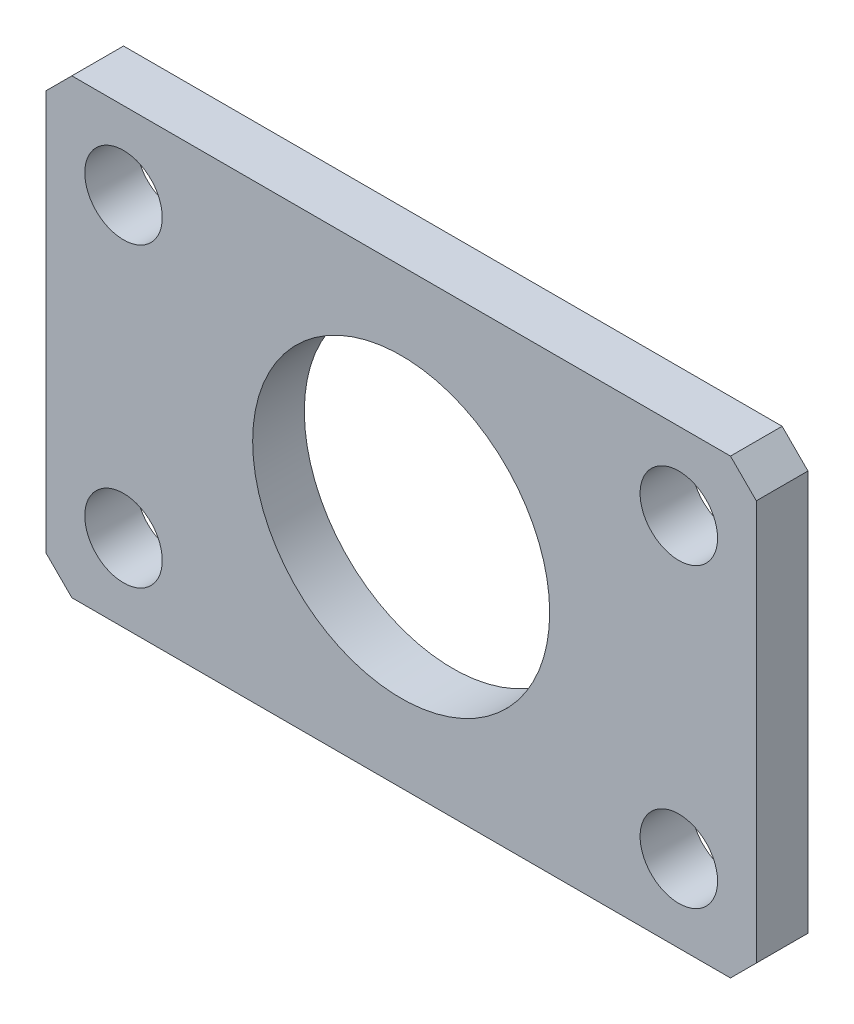
from build123d import *

# Parameters (mm, degrees)
SKETCH_1_W          = 55
SKETCH_1_H          = 35
SKETCH_1_R          = 11.5
EXTRUDE_1_DEPTH     = 2
CUT_EXTRUDE_1_REACH = 34.841
SKETCH_2_R          = 3
CHAMFER_1_SIZE      = 2


with BuildPart() as part:
    # 草图1 → 凸台-拉伸1 (new, symmetric)
    with BuildSketch(Plane.XY):
        Rectangle(SKETCH_1_W, SKETCH_1_H)
        Circle(SKETCH_1_R, mode=Mode.SUBTRACT)
    extrude(amount=EXTRUDE_1_DEPTH, both=True)

    # 草图2 → 切除-拉伸1 (cut, up to next)
    with BuildSketch(Plane.XY.offset(2), mode=Mode.PRIVATE) as cut_extrude_1_sk1:
        with Locations((-21.5, 11.5)):
            Circle(SKETCH_2_R)
    cut_extrude_1_tool1 = extrude(cut_extrude_1_sk1.sketch, amount=-CUT_EXTRUDE_1_REACH, mode=Mode.PRIVATE) & part.part
    # 草图2 → 切除-拉伸1 (cut, up to next)
    with BuildSketch(Plane.XY.offset(2), mode=Mode.PRIVATE) as cut_extrude_1_sk2:
        with Locations((21.5, 11.5)):
            Circle(SKETCH_2_R)
    cut_extrude_1_tool2 = extrude(cut_extrude_1_sk2.sketch, amount=-CUT_EXTRUDE_1_REACH, mode=Mode.PRIVATE) & part.part
    cut_extrude_1_1 = cut_extrude_1_tool1.solids().sort_by_distance((-21.5, 11.5, 2))[0]
    add(cut_extrude_1_1, mode=Mode.SUBTRACT)
    cut_extrude_1_2 = cut_extrude_1_tool2.solids().sort_by_distance((21.5, 11.5, 2))[0]
    add(cut_extrude_1_2, mode=Mode.SUBTRACT)
    cut_extrude_1 = cut_extrude_1_1 + cut_extrude_1_2  # 切除-拉伸1 as one shape, for the pattern or mirror that repeats it

    # 倒角1
    chamfer_1_edges = [part.edges().sort_by_distance(p)[0] for p in [
        (27.5, -17.5, 0),
        (-27.5, -17.5, 0),
        (-27.5, 17.5, 0),
        (27.5, 17.5, 0),
    ]]
    chamfer(chamfer_1_edges, length=CHAMFER_1_SIZE)

    # 镜向1: 切除-拉伸1 across plane
    add(cut_extrude_1.mirror(Plane.ZX), mode=Mode.SUBTRACT)


solid = part.part
